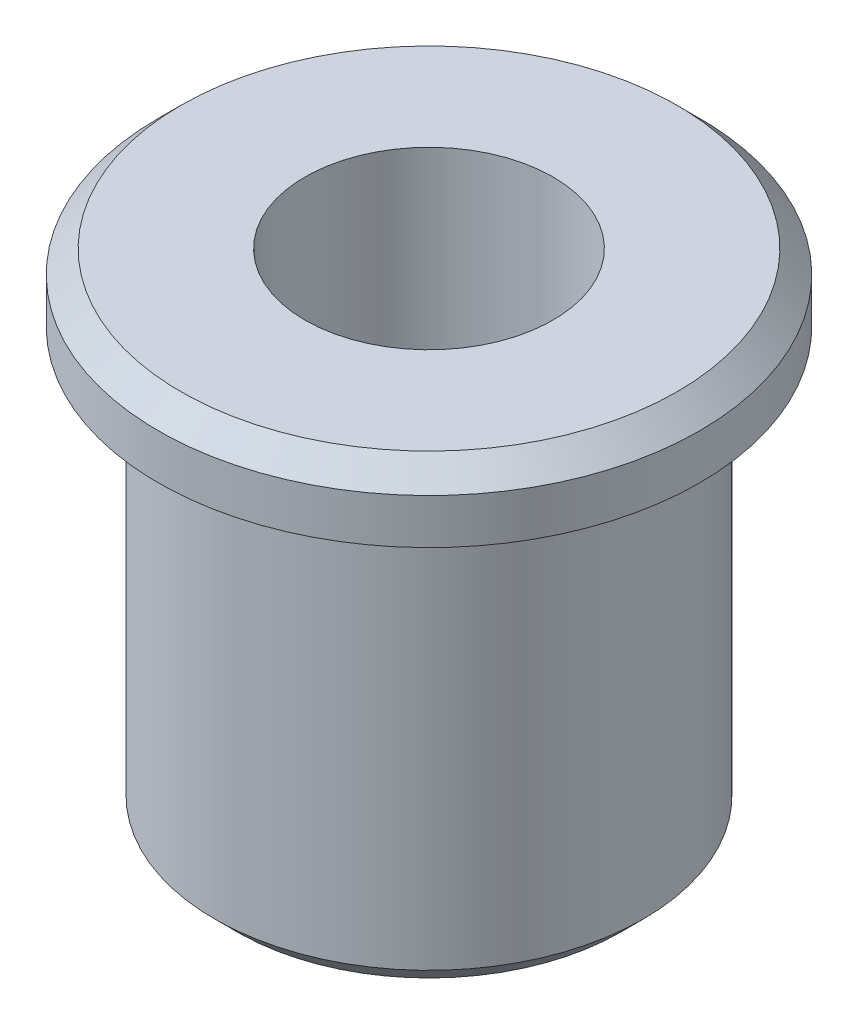
SolidWorks part; units mm, degrees
material "铜"
ref_plane "前视基准面" through (0, 0, 0) normal (0, 0, 1) x (1, 0, 0)
ref_plane "上视基准面" through (0, 0, 0) normal (0, 1, 0) x (1, 0, 0)
ref_plane "右视基准面" through (0, 0, 0) normal (1, 0, 0) x (0, 0, -1)
sketch "草图1" plane through (0, 0, 0) normal (0, 0, 1) x (1, 0, 0)
  line L0 (0, 0) -> (0, 22)
  line L1 (0, 22) -> (12, 22)
  line L2 (12, 22) -> (12, 19)
  line L3 (12, 19) -> (9.5, 19)
  line L4 (9.5, 19) -> (9.5, 0)
  line L5 (9.5, 0) -> (0, 0)
  dimension "D1" = 19
  dimension "D2" = 3
  dimension "D3" = 12
  dimension "D4" = 9.5
revolve "旋转1" add sketch "草图1" angle 360 about L0
sketch "草图2" plane through (0, 0, 0) normal (0, -1, 0) x (1, 0, 0)
  circle A0 centre (0, 0) radius 5.5
  dimension "D1" = 11
extrude "切除-拉伸1" cut sketch "草图2" against normal through all both
sketch "草图4" plane through (0, 0, 0) normal (0, -1, 0) x (1, 0, 0)
  circle A0 centre (0, 0) radius 5.25
  dimension "D1" = 10.5
chamfer "倒角1" distance 1 angle 45 1 edges at (12, 22, 0)
chamfer "倒角2" distance 1 angle 45 1 edges at (9.5, 0, 0)
